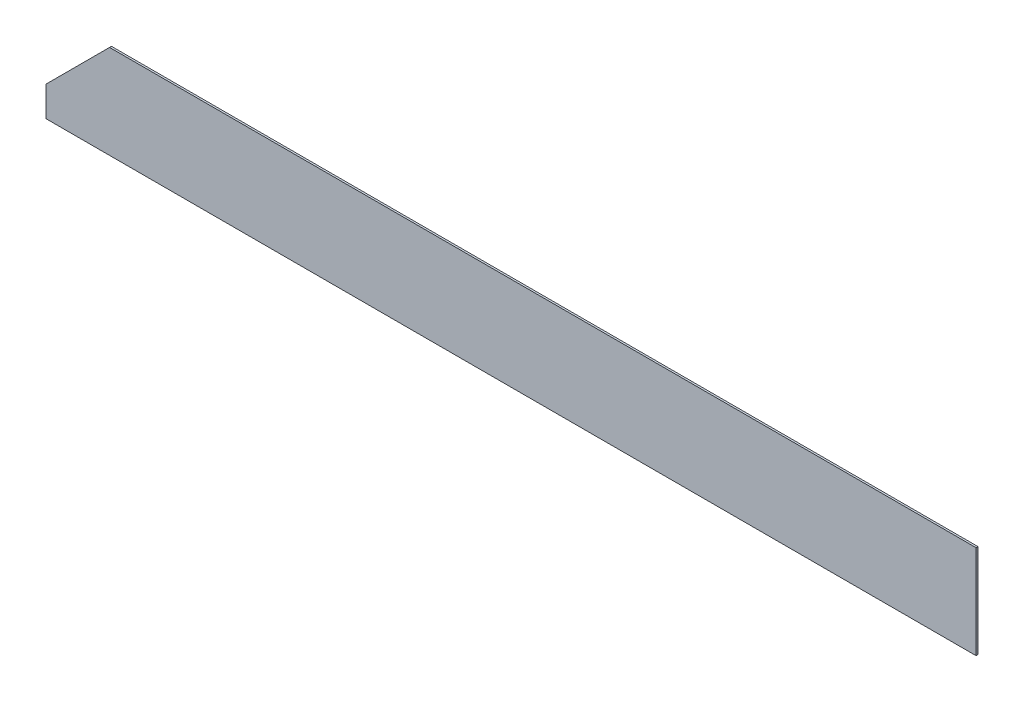
SolidWorks part; units mm, degrees
material "普通碳钢"
ref_plane "Front Plane" through (0, 0, 0) normal (0, 0, 1) x (1, 0, 0)
ref_plane "Top Plane" through (0, 0, 0) normal (0, 1, 0) x (1, 0, 0)
ref_plane "Right Plane" through (0, 0, 0) normal (1, 0, 0) x (0, 0, -1)
sketch "Sketch1" plane through (0, 0, 0) normal (0, 0, 1) x (1, 0, 0)
  line L0 (0, 0) -> (0, 780)
  line L1 (0, 780) -> (-7226, 780)
  line L2 (-7226, 780) -> (-7756, 250)
  line L3 (-7756, 250) -> (-7756, 0)
  line L4 (-7756, 0) -> (0, 0)
  dimension "D1" = 7756
  dimension "D2" = 780
  dimension "D3" = 250
  dimension "D4" = 45
extrude "Boss-Extrude1" add sketch "Sketch1" along normal mid plane 16
